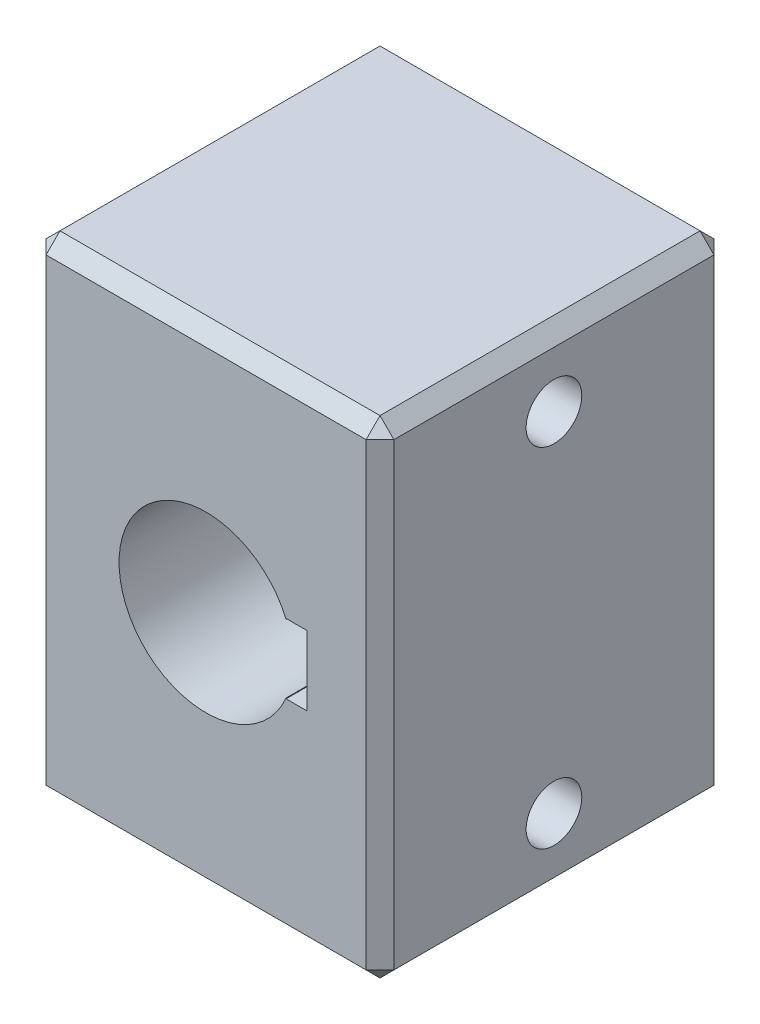
SolidWorks part; units mm, degrees
material "1060 合金"
ref_plane "前视基准面" through (0, 0, 0) normal (0, 0, 1) x (1, 0, 0)
ref_plane "上视基准面" through (0, 0, 0) normal (0, 1, 0) x (1, 0, 0)
ref_plane "右视基准面" through (0, 0, 0) normal (1, 0, 0) x (0, 0, -1)
sketch "草图1" plane through (0, 0, 0) normal (0, 0, 1) x (1, 0, 0)
  line L1 (-25, -35) -> (25, -35)
  line L2 (-25, -35) -> (-25, 35)
  line L3 (-25, 35) -> (25, 35)
  line L4 (25, -35) -> (25, 35)
  line L5 (-25, -35) -> (25, 35) construction
  line L6 (-25, 35) -> (25, -35) construction
  point P0 (0, 0)
  dimension "D1" = 50
  dimension "D2" = 70
extrude "凸台-拉伸1" add sketch "草图1" along normal blind 50
sketch "草图2" plane through (0, 0, 50) normal (0, 0, 1) x (1, 0, 0)
  circle A0 centre (0, 0) radius 12.5
  dimension "D1" = 25
extrude "切除-拉伸1" cut sketch "草图2" against normal through all
sketch "草图3" plane through (25, 0, 0) normal (1, 0, 0) x (0, 0, -1)
  circle A0 centre (-15, 0) radius 4.6612
sketch "草图12" plane through (25, 0, 0) normal (1, 0, 0) x (0, 0, -1)
  circle A0 centre (-25, 25) radius 4
  dimension "D2" = 8
extrude "切除-拉伸5" cut sketch "草图12" against normal blind 58
mirror "镜向1" about plane through (0, 0, 0) normal (0, 1, 0) of "切除-拉伸5"
chamfer "倒角1" distance 2 angle 45 12 edges at (0, 35, 0) (-25, 0, 0) (25, 0, 0) (-25, -35, 25) (0, -35, 50) (0, -35, 0) (25, -35, 25) (-25, 0, 50) (25, 0, 50) (-25, 35, 25) (0, 35, 50) (25, 35, 25)
sketch "草图13" plane through (25, 0, 0) normal (1, 0, 0) x (0, 0, -1)
  line L0 (-50, 0) -> (-28, 0) construction
  line L1 (-50, 5) -> (-28, 5)
  line L2 (-50, -5) -> (-28, -5)
  line L4 (-50, -33) -> (-50, 33) construction
  arc A0 (-50, 5) -> (-50, -5) centre (-50, 0) ccw
  arc A1 (-28, -5) -> (-28, 5) centre (-28, 0) ccw
  point P2 (-39, 0)
  dimension "D3" = 32
  dimension "D1" = 10
extrude "切除-拉伸6" cut sketch "草图13" along normal blind 3 from offset 13.5
